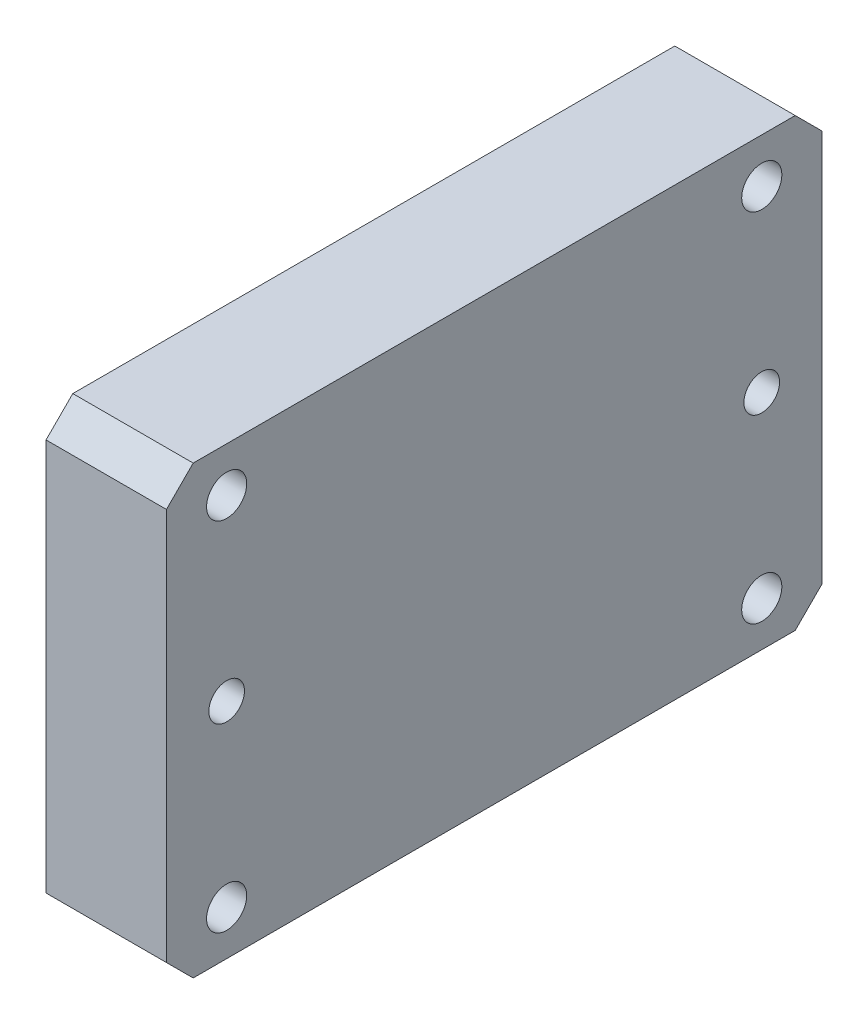
SolidWorks part; units mm, degrees
material "AL6061"
ref_plane "Front Plane" through (0, 0, 0) normal (0, 0, 1) x (1, 0, 0)
ref_plane "Top Plane" through (0, 0, 0) normal (0, 1, 0) x (1, 0, 0)
ref_plane "Right Plane" through (0, 0, 0) normal (1, 0, 0) x (0, 0, -1)
sketch "Sketch1" plane through (0, 0, 0) normal (1, 0, 0) x (0, 0, -1)
  line L1 (-36.75, -25) -> (36.75, -25)
  line L2 (-36.75, -25) -> (-36.75, 25)
  line L3 (-36.75, 25) -> (36.75, 25)
  line L4 (36.75, -25) -> (36.75, 25)
  line L5 (-36.75, -25) -> (36.75, 25) construction
  line L6 (-36.75, 25) -> (36.75, -25) construction
  point P0 (0, 0)
  dimension "D1" = 73.5
  dimension "D2" = 50
extrude "Boss-Extrude1" add sketch "Sketch1" along normal blind 13.5
hole_wizard "CBORE for M4 Hexagon socket head cap screws1" positions "Sketch2" profile "Sketch3" counterbore size "M4" standard "GB" end condition through all
sketch "Sketch2" plane through (0, 0, 0) normal (-1, 0, 0) x (0, 0, 1)
  line L0 (36.75, 0) -> (0, 0) construction
  line L1 (36.75, 25) -> (36.75, -25) construction
  line L3 (0, 0) -> (0, 25) construction
  line L4 (-36.75, 25) -> (36.75, 25) construction
  point P14 (30, 20)
  point P16 (-30, 20)
  point P20 (-30, -20)
  point P21 (30, -20)
  dimension "D1" = 60
  dimension "D2" = 40
sketch "Sketch3" plane through (0, -20, 30) normal (0, 1, 0) x (0, 0, 1)
  line L0 (0, 0) -> (0, 13.5)
  line L1 (0, 13.5) -> (2.25, 13.5)
  line L3 (2.25, 13.5) -> (2.25, 4.6)
  line L4 (2.25, 4.6) -> (4, 4.6)
  line L5 (4, 4.6) -> (4, 0)
  line L7 (4, 0) -> (0, 0)
  line L11 (0, -6.35) -> (0, 107.95) construction
  dimension "通孔孔直径" = 4.5
  dimension "通孔孔深度" = 13.5
  dimension "柱形沉头孔直径" = 8
  dimension "柱形沉头孔深度" = 4.6
hole_wizard "Ø4.0mm Dowel Hole1" positions "Sketch4" profile "Sketch5" hole size "Ø4.0" standard "GB"
sketch "Sketch4" plane through (13.5, 0, 0) normal (1, 0, 0) x (0, 0, -1)
  line L0 (-30, 20) -> (-30, -20) construction
  line L2 (30, 20) -> (30, -20) construction
  point P12 (-30, 0)
  point P14 (30, 0)
sketch "Sketch5" plane through (13.5, 0, -30) normal (0, 1, 0) x (0, 0, -1)
  line L0 (0, 0) -> (0, 7.2017)
  line L1 (0, 7.2017) -> (2, 6)
  line L2 (2, 6) -> (2, 0)
  line L5 (2, 0) -> (0, 0)
  line L10 (0, 7.2017) -> (-2, 6) construction
  line L11 (0, -6.35) -> (0, 107.95) construction
  dimension "孔直径" = 4
  dimension "孔深度" = 6
  dimension "导头角度" = 118
hole_wizard "M4 Tapped Hole1" positions "Sketch6" profile "Sketch7" tap size "M4" standard "GB"
sketch "Sketch6" plane through (0, 0, 0) normal (-1, 0, 0) x (0, 0, 1)
  point P0 (28.25, -11.25)
  point P3 (-30.75, -11.25)
sketch "Sketch7" plane through (0, -11.25, 28.25) normal (0, 1, 0) x (0, 0, 1)
  line L0 (0, 0) -> (0, 11.0914)
  line L1 (0, 11.0914) -> (1.65, 10.1)
  line L2 (1.65, 10.1) -> (1.65, 0)
  line L5 (1.65, 0) -> (0, 0)
  line L10 (0, 11.0914) -> (-1.65, 10.1) construction
  line L11 (0, -6.35) -> (0, 107.95) construction
  dimension "螺纹孔钻头直径" = 3.3
  dimension "螺纹孔钻头深度" = 10.1
  dimension "导头角度" = 118
cosmetic thread "Cosmetic Thread1" parameters "D1"=8, "D2"=4
cosmetic thread "Cosmetic Thread2" parameters "D1"=8, "D2"=4
chamfer "Chamfer1" distance 3 angle 45 4 edges at (6.75, -25, -36.75) (6.75, 25, -36.75) (6.75, -25, 36.75) (6.75, 25, 36.75)
